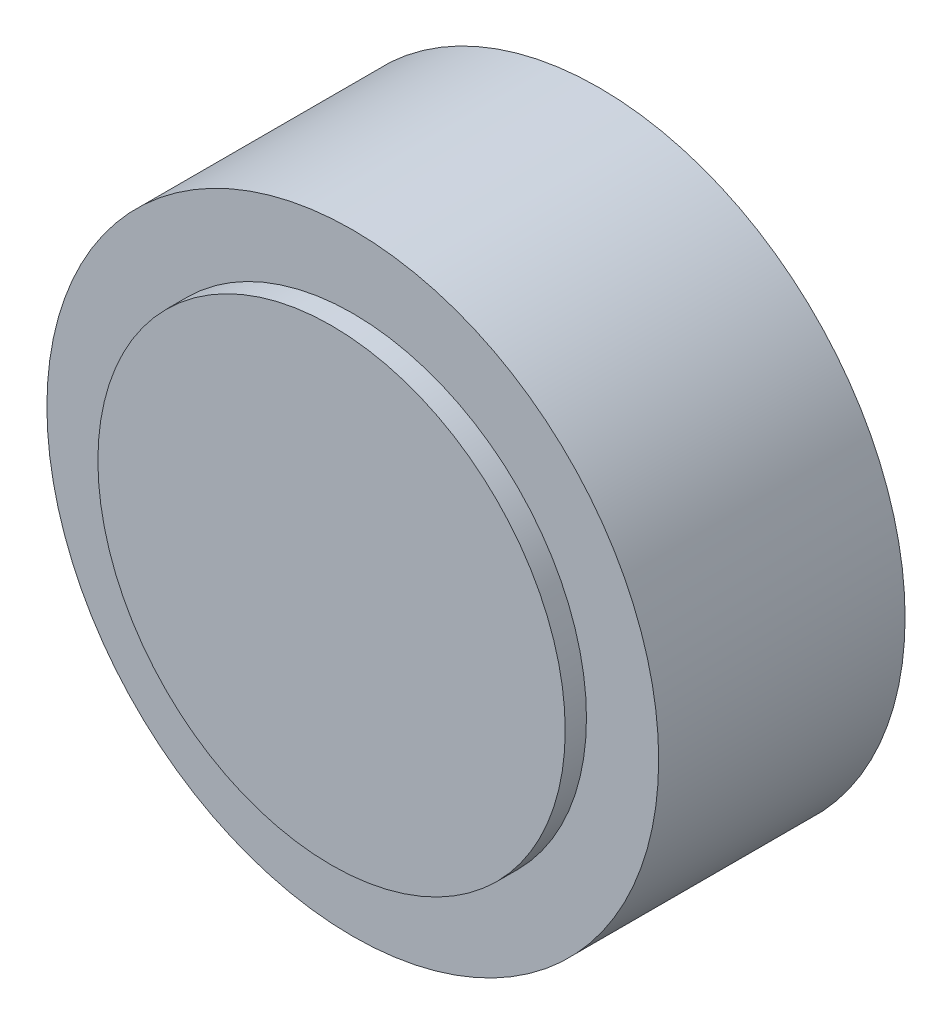
SolidWorks part; units mm, degrees
material "普通碳钢"
ref_plane "Front Plane" through (0, 0, 0) normal (0, 0, 1) x (1, 0, 0)
ref_plane "Top Plane" through (0, 0, 0) normal (0, 1, 0) x (1, 0, 0)
ref_plane "Right Plane" through (0, 0, 0) normal (1, 0, 0) x (0, 0, -1)
sketch "Sketch1" plane through (0, 0, 0) normal (0, 0, 1) x (1, 0, 0)
  circle A0 centre (0, 0) radius 72
  dimension "D1" = 144
extrude "Boss-Extrude1" add sketch "Sketch1" along normal blind 58
sketch "Sketch2" plane through (0, 0, 58) normal (0, 0, 1) x (1, 0, 0)
  circle A0 centre (0, 0) radius 55
  dimension "D1" = 110
extrude "Boss-Extrude2" add sketch "Sketch2" along normal blind 5
